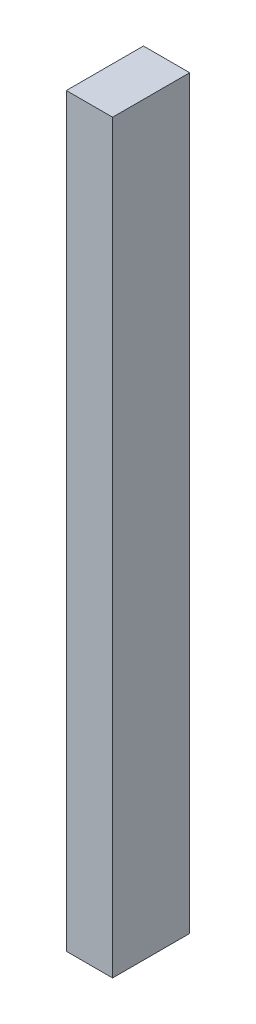
from build123d import *

# Parameters (mm, degrees)
SKETCH_1_W      = 30
SKETCH_1_H      = 483.5
EXTRUDE_1_DEPTH = 50


with BuildPart() as part:
    # 草图1 → 凸台-拉伸1 (new body)
    with BuildSketch(Plane.XY):
        Rectangle(SKETCH_1_W, SKETCH_1_H)
    extrude(amount=EXTRUDE_1_DEPTH)


solid = part.part
